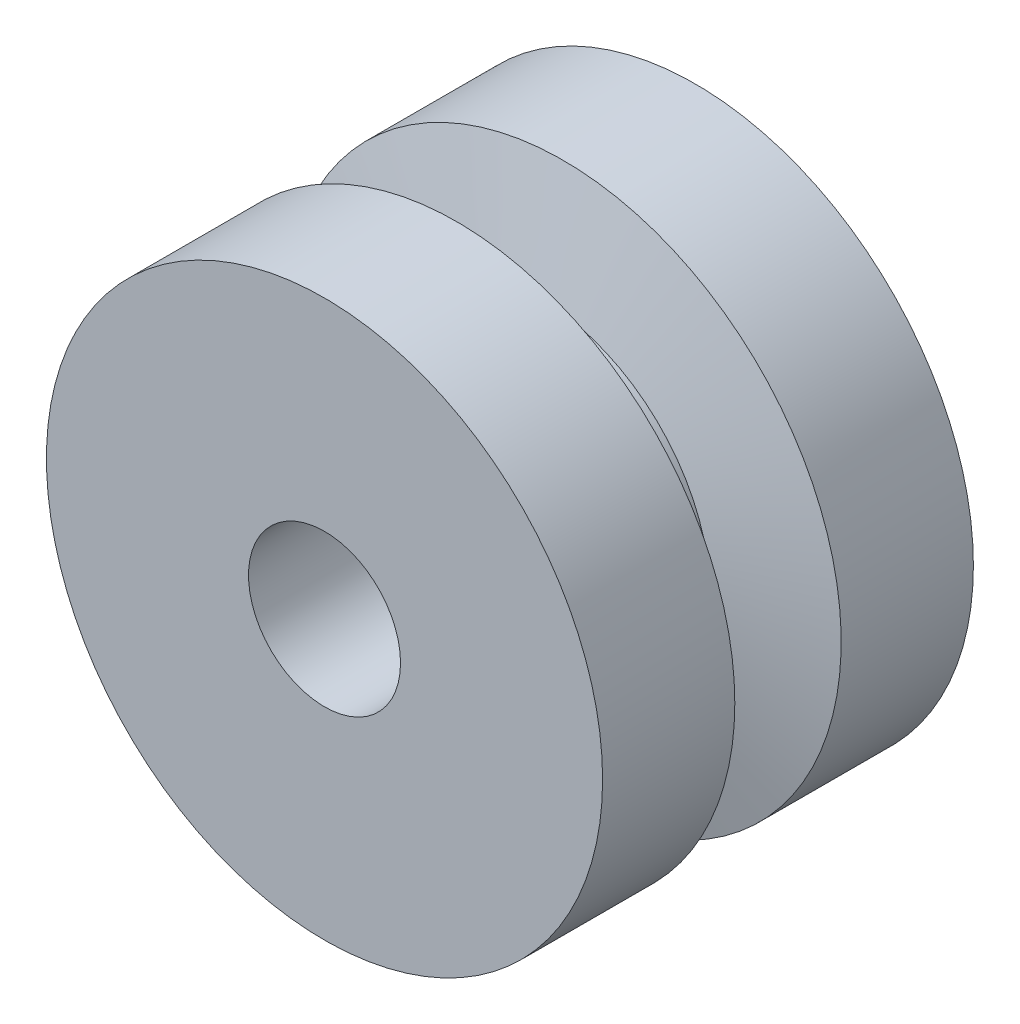
from build123d import *

# Parameters (mm, degrees)
SKETCH_1_R      = 37.5
SKETCH_1_R_2    = 10.25
EXTRUDE_1_DEPTH = 50


with BuildPart() as part:
    # 草图1 → 凸台-拉伸1 (new body)
    with BuildSketch(Plane.XY):
        Circle(SKETCH_1_R)
        Circle(SKETCH_1_R_2, mode=Mode.SUBTRACT)
    extrude(amount=EXTRUDE_1_DEPTH)

    # 草图2 → 切除-旋转1 (revolve, cut)
    with BuildSketch(Plane(origin=(0, 0, 0), x_dir=(1, 0, 0), z_dir=(0, 1, 0))):
        Polygon((-38.25, -17.648818614), (-23.25, -21.25), (-23.25, -28.75), (-38.25, -32.351181386), align=None)
    revolve(axis=Axis((0, 0, 0), (0, 0, 1)), mode=Mode.SUBTRACT)

    # 草图3 → M5 螺纹孔2 (revolve, cut)
    with BuildSketch(Plane(origin=(0, 32.5, 9), x_dir=(0, 0, 1), z_dir=(1, 0, 0))):
        Polygon((0, 0), (0, 31.2618073), (2.1, 30), (2.1, 0), align=None)
    revolve(axis=Axis((0, 38.85, 9), (0, -1, 0)), mode=Mode.SUBTRACT)

    # 草图5 → M5 螺纹孔1 (revolve, cut)
    with BuildSketch(Plane(origin=(32.5, 0, 9), x_dir=(0, 0, -1), z_dir=(0, 1, 0))):
        Polygon((0, 0), (0, 31.2618073), (2.1, 30), (2.1, 0), align=None)
    revolve(axis=Axis((38.85, 0, 9), (-1, 0, 0)), mode=Mode.SUBTRACT)


solid = part.part
